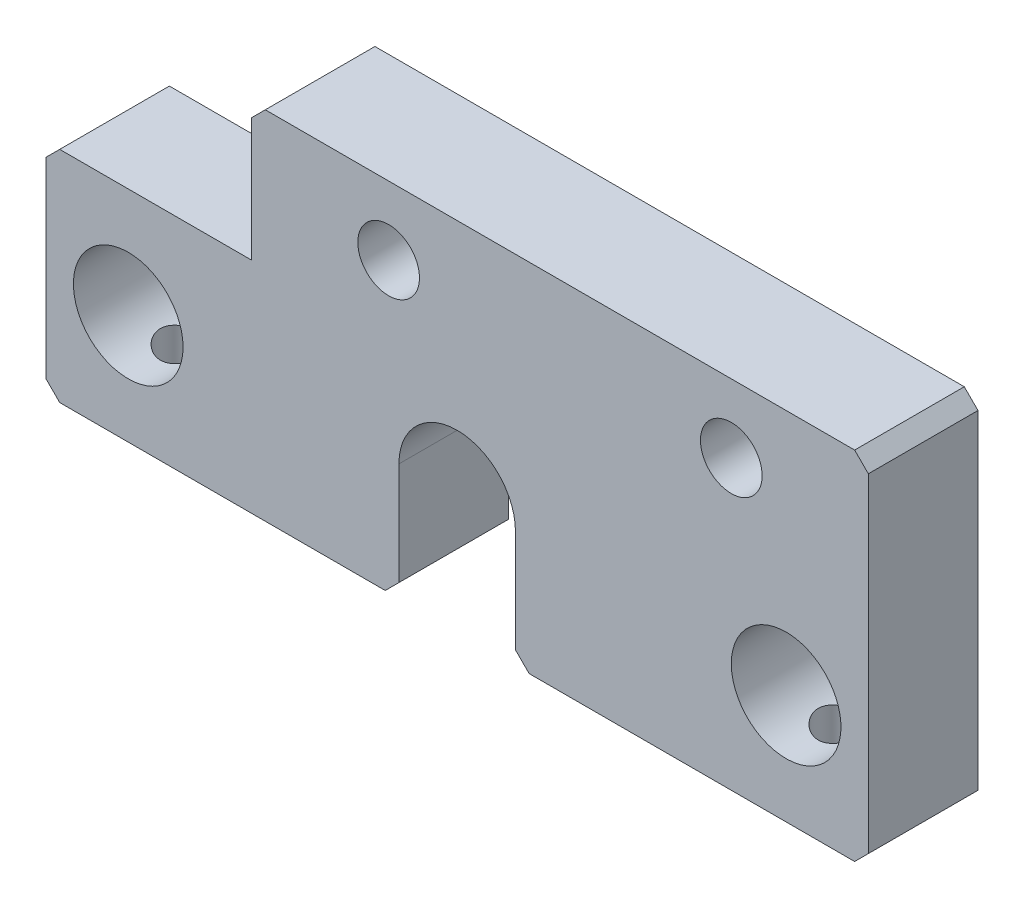
SolidWorks part; units mm, degrees
material "S45C"
ref_plane "Front Plane" through (0, 0, 0) normal (0, 0, 1) x (1, 0, 0)
ref_plane "Top Plane" through (0, 0, 0) normal (0, 1, 0) x (1, 0, 0)
ref_plane "Right Plane" through (0, 0, 0) normal (1, 0, 0) x (0, 0, -1)
sketch "Sketch1" plane through (0, 0, 0) normal (0, 0, 1) x (1, 0, 0)
  line L0 (0, 0) -> (0, 28.708) construction
  line L1 (30, 0) -> (-30, 0)
  line L2 (30, 0) -> (30, 26)
  line L3 (30, 26) -> (-30, 26)
  line L4 (-30, 0) -> (-30, 26)
  circle A0 centre (-24, 8) radius 4
  circle A1 centre (24, 8) radius 4
  dimension "D3" = 8
  dimension "D4" = 48
  dimension "D5" = 8
  dimension "D1" = 60
  dimension "D2" = 26
extrude "Boss-Extrude1" add sketch "Sketch1" along normal blind 8
sketch "Sketch2" plane through (0, 0, 8) normal (0, 0, 1) x (1, 0, 0)
  line L0 (0, 0) -> (0, 8.5) construction
  line L1 (-4.25, 0) -> (-4.25, 8.5)
  line L2 (4.25, 0) -> (4.25, 8.5)
  arc A0 (-4.25, 0) -> (4.25, 0) centre (0, 0) ccw
  arc A1 (4.25, 8.5) -> (-4.25, 8.5) centre (0, 8.5) ccw
  point P3 (0, 4.25)
  dimension "D1" = 4.25
  dimension "D2" = 8.5
extrude "Cut-Extrude1" cut sketch "Sketch2" against normal through all
hole_wizard "M4 Tapped Hole1" positions "Sketch4" profile "Sketch5" tap size "M4" standard "GB"
sketch "Sketch4" plane through (0, 0, 0) normal (0, -1, 0) x (1, 0, 0)
  line L0 (30, 4) -> (24, 4) construction
  line L1 (30, 8) -> (30, 0) construction
  line L2 (24, 4) -> (-24, 4) construction
  point P0 (-24, 4)
  point P1 (24, 4)
  dimension "D1" = 48
  dimension "D2" = 24
sketch "Sketch5" plane through (-24, 0, 4) normal (1, 0, 0) x (0, 0, -1)
  line L0 (0, 0) -> (0, 4)
  line L1 (0, 4) -> (1.65, 4)
  line L2 (1.65, 4) -> (1.65, 0)
  line L5 (1.65, 0) -> (0, 0)
  line L11 (0, -6.35) -> (0, 107.95) construction
  dimension "通孔螺纹孔钻头直径" = 3.3
  dimension "通孔螺纹孔钻头深度" = 4
cosmetic thread "Cosmetic Thread 1" parameters "D2"=4
cosmetic thread "Cosmetic Thread 2" parameters "D2"=4
hole_wizard "Hole size per hex socket cap screw type 1" positions "Sketch7" profile "Sketch6" counterbore size "M4" standard "GB"
sketch "Sketch7" plane through (-35.6709, -1.9786, 0) normal (0, 0, 1) x (1, 0, 0)
  line L0 (15.6709, 32.9786) -> (40.6709, 32.9786) construction
  line L3 (65.6709, 37.9786) -> (5.6709, 37.9786) construction
  line L4 (5.6709, 37.9786) -> (5.6709, 2.9786) construction
  point P0 (40.6709, 32.9786)
  point P1 (15.6709, 32.9786)
  dimension "D1" = 25
  dimension "D2" = 10
  dimension "D3" = 5
sketch "Sketch6" plane through (5, 31, 0) normal (1, 0, 0) x (0, 1, 0)
  line L0 (0, 0) -> (0, 8)
  line L1 (0, 8) -> (2.25, 8)
  line L3 (2.25, 8) -> (2.25, 4.6)
  line L4 (2.25, 4.6) -> (4, 4.6)
  line L5 (4, 4.6) -> (4, 0)
  line L7 (4, 0) -> (0, 0)
  line L11 (0, -6.35) -> (0, 107.95) construction
  dimension "通孔孔直径" = 4.5
  dimension "通孔孔深度" = 8
  dimension "柱形沉头孔直径" = 8
  dimension "柱形沉头孔深度" = 4.6
sketch "Sketch8" plane through (0, 0, 0) normal (0, 0, -1) x (-1, 0, 0)
  line L1 (15, 26) -> (30, 26)
  line L2 (15, 26) -> (15, 16)
  line L3 (15, 16) -> (30, 16)
  line L4 (30, 26) -> (30, 16)
  dimension "D1" = 15
  dimension "D2" = 10
extrude "Cut-Extrude2" cut sketch "Sketch8" against normal through all
sketch "Sketch9" plane through (0, 0, 0) normal (0, 0, -1) x (-1, 0, 0)
  line L0 (30, 21) -> (-15, 21) construction
  line L1 (30, 16) -> (30, 0) construction
  line L2 (15, 26) -> (15, 16) construction
  line L9 (-30, 26) -> (15, 26) construction
  circle A4 centre (-20, 21) radius 2.25
  circle A5 centre (5, 21) radius 2.25
  dimension "D6" = 4.5
  dimension "D1" = 25
  dimension "D2" = 10
  dimension "D5" = 5
extrude "Cut-Extrude3" cut sketch "Sketch9" against normal through all
chamfer "Chamfer1" distance 1 angle 45 7 edges at (30, 0, 4) (-30, 0, 4) (4.25, 0, 4) (-4.25, 0, 4) (30, 26, 4) (-15, 26, 4) (-30, 16, 4)
